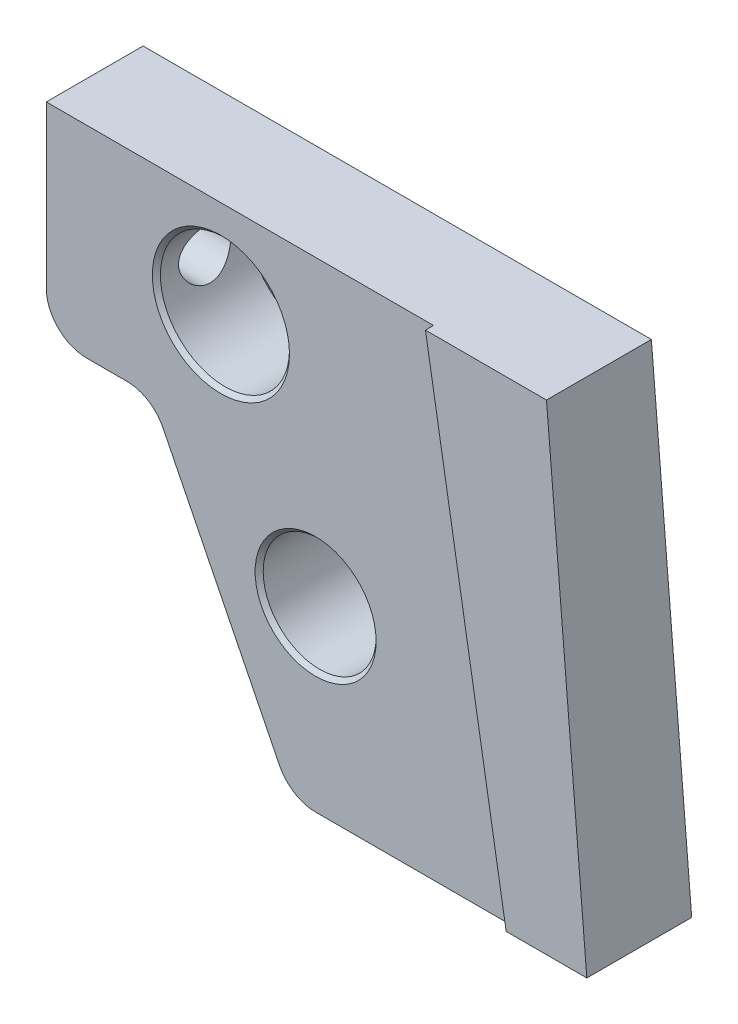
from build123d import *

# Parameters (mm, degrees)
SKETCH1_R           = 8
SKETCH1_R_2         = 7
BOSS_EXTRUDE1_DEPTH = 13
CUT_EXTRUDE1_START  = -1
CUT_EXTRUDE1_DEPTH  = 1
CHAMFER2_SIZE       = 0.5
SKETCH3_R           = 3.25
CUT_EXTRUDE2_DEPTH  = 17


with BuildPart() as part:
    # Sketch1 → Boss-Extrude1 (new body)
    with BuildSketch(Plane.XY):
        with BuildLine():
            Line((0, 5), (0, 25))
            Line((0, 25), (63, 25))
            Line((63, 25), (68, -34.543411946))
            Line((68, -34.543411946), (33.385133941, -34.543411946))
            ThreePointArc((33.385133941, -34.543411946), (30.752722356, -33.794342344), (28.909054571, -31.771575646))
            Line((28.909054571, -31.771575646), (14.473169684, -2.7718363))
            ThreePointArc((14.473169684, -2.7718363), (12.629501898, -0.749069602), (9.997090314, 0))
            Line((9.997090314, 0), (5, 0))
            ThreePointArc((5, 0), (1.464466094, 1.464466094), (0, 5))
        make_face()
        with Locations(Location((21.645133941, 13, 0), (0, 0, 180))):
            Circle(SKETCH1_R, mode=Mode.SUBTRACT)
        with Locations(Location((33.385133941, -12.47, 0), (0, 0, 180))):
            Circle(SKETCH1_R_2, mode=Mode.SUBTRACT)
    extrude(amount=BOSS_EXTRUDE1_DEPTH)

    # Sketch2 → Cut-Extrude1 (cut)
    with BuildSketch(Plane.XY.offset(13).offset(CUT_EXTRUDE1_START)):
        with BuildLine():
            Line((48, 25), (58, -34.543411946))
            Line((58, -34.543411946), (33.385133941, -34.543411946))
            ThreePointArc((33.385133941, -34.543411946), (30.752722356, -33.794342344), (28.909054571, -31.771575646))
            Line((28.909054571, -31.771575646), (14.473169684, -2.7718363))
            ThreePointArc((14.473169684, -2.7718363), (12.629501898, -0.749069602), (9.997090314, 0))
            Line((9.997090314, 0), (5, 0))
            ThreePointArc((5, 0), (1.464466094, 1.464466094), (0, 5))
            Line((0, 5), (0, 25))
            Line((0, 25), (48, 25))
        make_face()
    extrude(amount=CUT_EXTRUDE1_DEPTH, mode=Mode.SUBTRACT)

    # Chamfer2
    chamfer2_edges = [part.edges().sort_by_distance(p)[0] for p in [
        (29.645133941, 13, 0),
        (40.385133941, -12.47, 0),
        (29.645133941, 13, 12),
        (40.385133941, -12.47, 12),
    ]]
    chamfer(chamfer2_edges, length=CHAMFER2_SIZE)

    # Sketch3 → Cut-Extrude2 (cut)
    with BuildSketch(Plane.ZY):
        with Locations((6, 13)):
            Circle(SKETCH3_R)
    extrude(amount=-CUT_EXTRUDE2_DEPTH, mode=Mode.SUBTRACT)


solid = part.part
